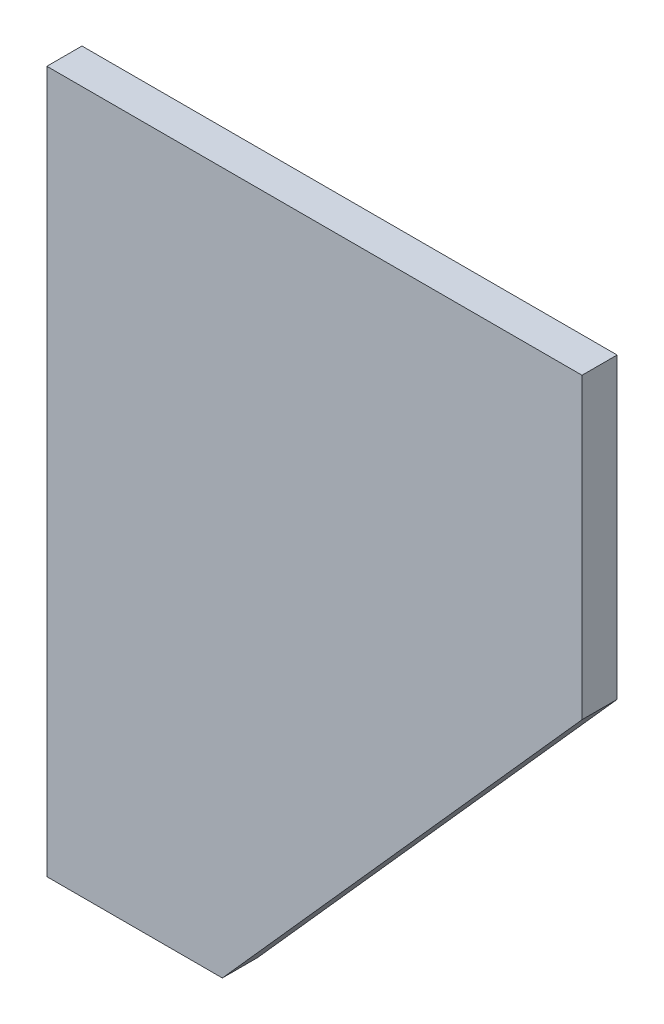
SolidWorks part; units mm, degrees
material "普通碳钢"
ref_plane "前视基准面" through (0, 0, 0) normal (0, 0, 1) x (1, 0, 0)
ref_plane "上视基准面" through (0, 0, 0) normal (0, 1, 0) x (1, 0, 0)
ref_plane "右视基准面" through (0, 0, 0) normal (1, 0, 0) x (0, 0, -1)
sketch "草图1" plane through (0, 0, 0) normal (0, 0, 1) x (1, 0, 0)
  line L0 (0, 0) -> (30.5, 0)
  line L1 (30.5, 0) -> (30.5, -17)
  line L2 (30.5, -17) -> (10, -40)
  line L3 (10, -40) -> (0, -40)
  line L4 (0, -40) -> (0, 0)
  dimension "D1" = 30.5
  dimension "D2" = 40
  dimension "D3" = 17
  dimension "D4" = 10
extrude "凸台-拉伸1" add sketch "草图1" along normal blind 2
equation "\"Bh\"= \"D1@凸台-拉伸1\""
